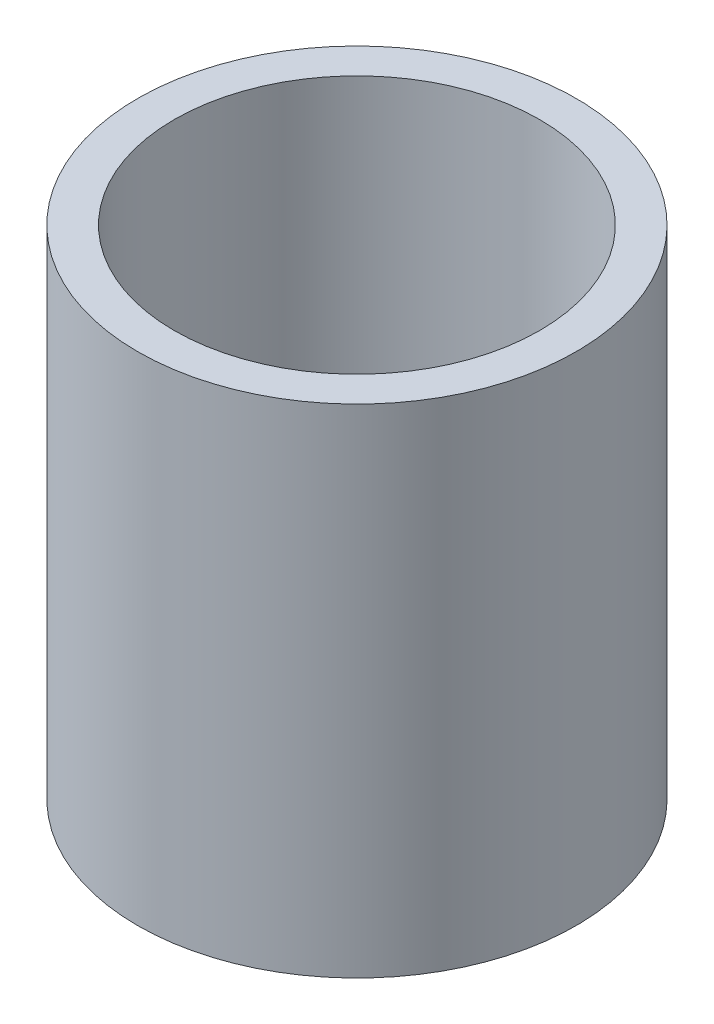
from build123d import *

# Parameters (mm, degrees)
SKETCH_1_R      = 15
SKETCH_1_R_2    = 12.5
EXTRUDE_1_DEPTH = 34


with BuildPart() as part:
    # 草图1 → 凸台-拉伸1 (new body)
    with BuildSketch(Plane(origin=(0, 0, 0), x_dir=(1, 0, 0), z_dir=(0, 1, 0))):
        with Locations(Location((0, 0, 0), (0, 0, 270))):
            Circle(SKETCH_1_R)
        with Locations(Location((0, 0, 0), (0, 0, 270))):
            Circle(SKETCH_1_R_2, mode=Mode.SUBTRACT)
    extrude(amount=EXTRUDE_1_DEPTH)


solid = part.part
